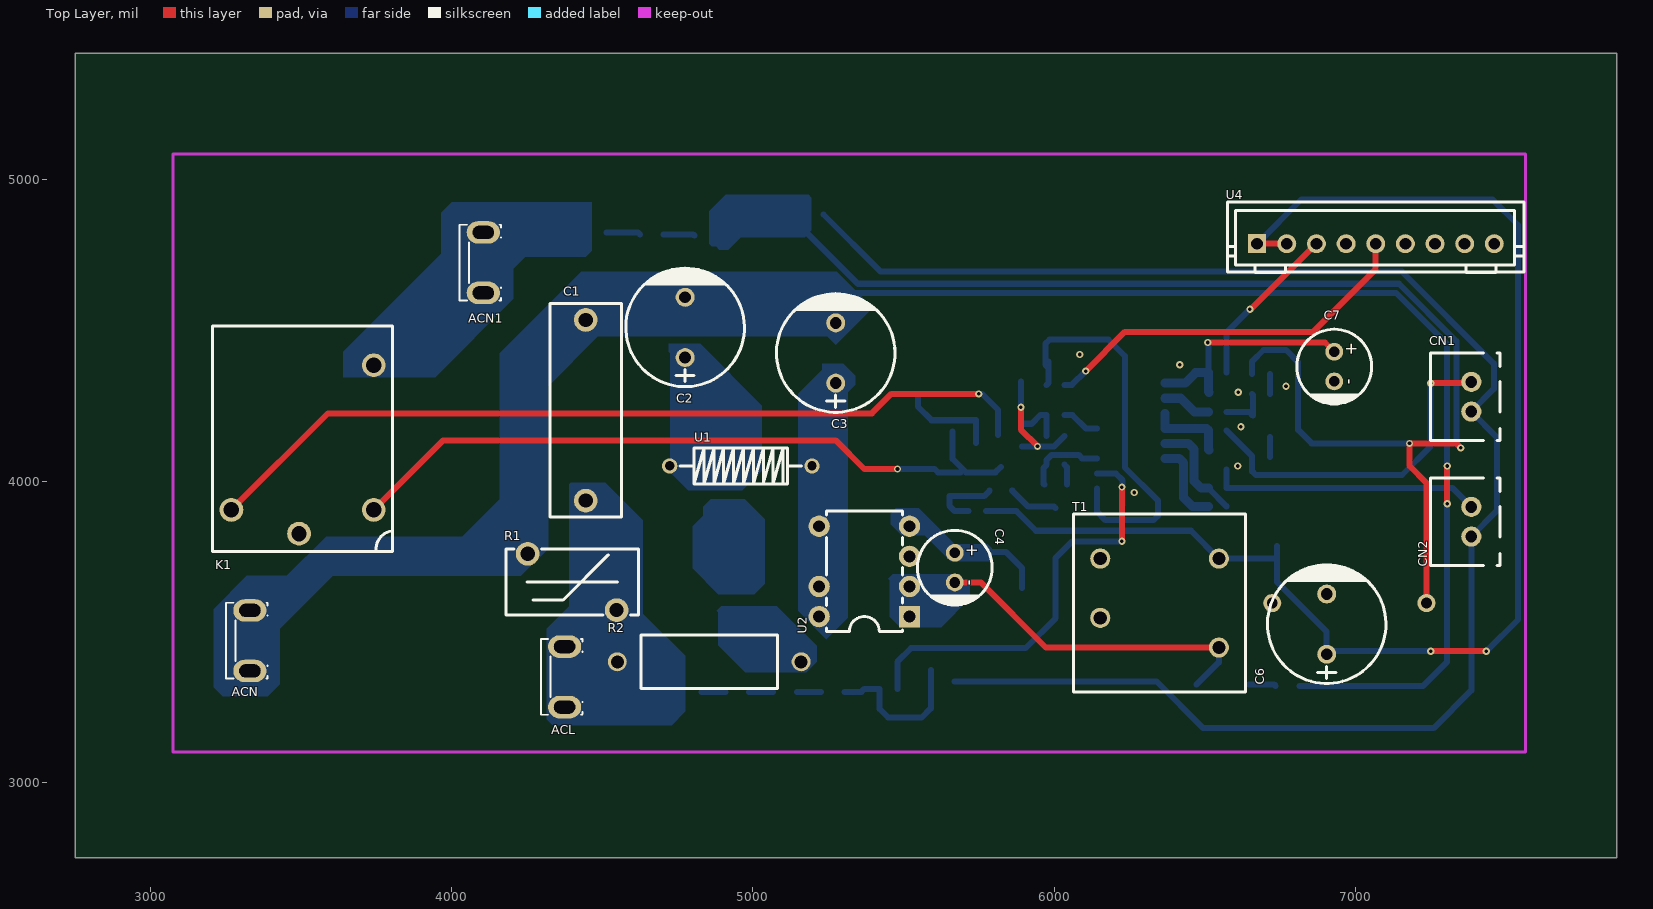
[diagram p0: Top Layer view]
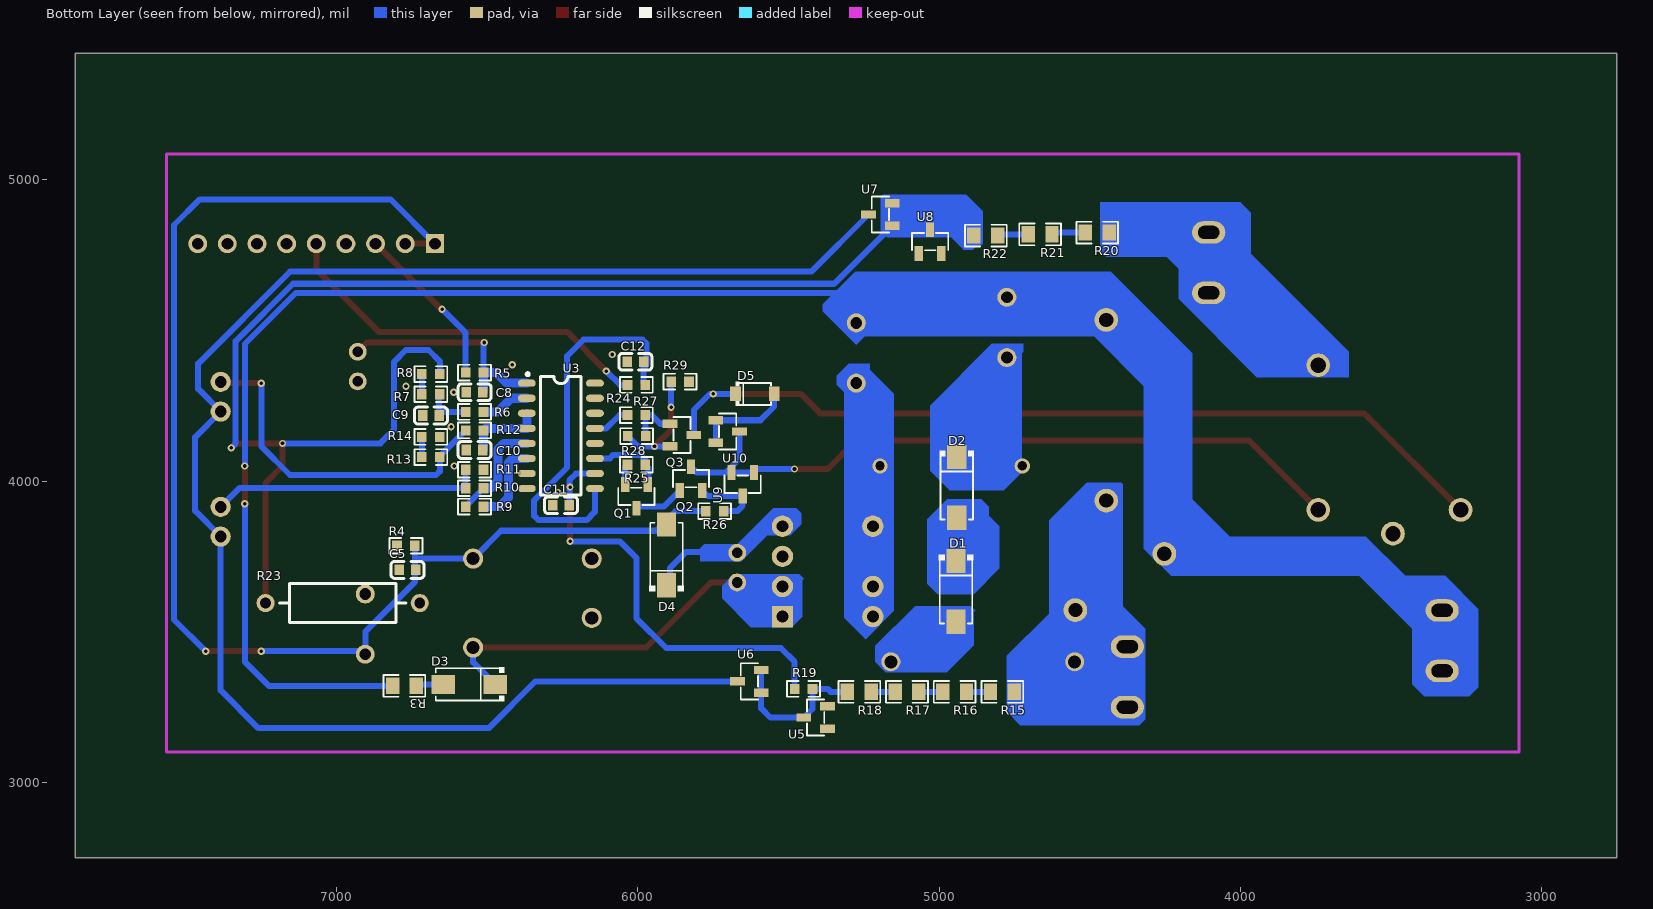
[diagram p1: Bottom Layer view, seen from below]
# Altium PCB MISC51809.pcbdoc
Units mil, origin at the board's own origin, x right, y up, seen from the top; angles counter-clockwise.
Board outline 5118.18 x 2670.55 mil, 2 copper layers (Top Layer, Bottom Layer), stack 62.206 mil thick; 66 components, 45 nets, 171 pads, 23 vias.

## Layer stack, top to bottom
Top Solder Mask Layer: solder mask 0.394, Dk 3.3
Top Layer: signal copper 1.379
Dielectric1: surface 59.449, FR4, Dk 4.5
Bottom Layer: signal copper 1.378
Bottom Solder Mask Layer: solder mask 0.394, Dk 3.3

## Board outline
7868.18,2750 2750,2750 2750,5420.55 7868.18,5420.55

## Design rules (kind name [scope] priority, off if disabled: settings)
BoardOutlineClearance copperThickness2oz_1 [All] p2 off: genericclearance=7.99 ignorepadtopadclearanceinfootprint=FALSE except(0: Arc-SplitContinuation Track-SplitContinuation SMDPad-SplitContinuation THPad-SplitContinuation Via-SplitContinuation Fill-SplitContinuation Region-SplitContinuation Poly-SplitContinuation Text-SplitContinuation Hole-SplitContinuation; 5.98: Arc-CutoutEdge SMDPad-CutoutEdge THPad-CutoutEdge Via-CutoutEdge Fill-CutoutEdge Region-CutoutEdge Text-CutoutEdge; 6.93: Hole-OutlineEdge Hole-CutoutEdge; 10: Poly-OutlineEdge Poly-CutoutEdge; 11.81: Arc-OutlineEdge Track-OutlineEdge SMDPad-OutlineEdge THPad-OutlineEdge Via-OutlineEdge Fill-OutlineEdge Region-OutlineEdge Text-OutlineEdge Track-CutoutEdge)
BoardOutlineClearance copperThickness1oz_1 [All] p4: genericclearance=4.02 ignorepadtopadclearanceinfootprint=FALSE except(0: Arc-SplitContinuation Track-SplitContinuation SMDPad-SplitContinuation THPad-SplitContinuation Via-SplitContinuation Fill-SplitContinuation Region-SplitContinuation Poly-SplitContinuation Text-SplitContinuation Hole-SplitContinuation; 6: SMDPad-CutoutEdge THPad-CutoutEdge Via-CutoutEdge Fill-CutoutEdge Region-CutoutEdge Text-CutoutEdge; 6.93: Hole-OutlineEdge Hole-CutoutEdge; 10: Poly-OutlineEdge Poly-CutoutEdge; 11.8: Arc-OutlineEdge Track-OutlineEdge SMDPad-OutlineEdge THPad-OutlineEdge Via-OutlineEdge Fill-OutlineEdge Region-OutlineEdge Text-OutlineEdge; 11.81: Arc-CutoutEdge Track-CutoutEdge)
Clearance copperThickness2oz [All] p1 off: gap=7.99 ignorepadtopadclearanceinfootprint=FALSE except(5.98: SMDPad-Track SMDPad-SMDPad THPad-Track SMDPad-THPad THPad-THPad Track-Via SMDPad-Via THPad-Via Via-Via Fill-Track Region-Track Fill-SMDPad Region-SMDPad Fill-THPad Region-THPad Fill-Via Region-Via Fill-Fill Fill-Region Region-Region Arc-Track Arc-SMDPad Arc-THPad Arc-Via Fill-Arc Region-Arc Arc-Arc Text-Track SMDPad-Text Text-THPad Text-Via Fill-Text Region-Text Arc-Text Text-Text; 6.93: Hole-Track Hole-SMDPad Hole-THPad Hole-Via Fill-Hole Region-Hole Hole-Arc Hole-Text; 10: Poly-Track Poly-SMDPad Poly-THPad Poly-Via Poly-Fill Poly-Region Poly-Poly Poly-Arc Poly-Text Poly-Hole)
Clearance copperThickness1oz [All] p3: gap=4.02 ignorepadtopadclearanceinfootprint=FALSE except(5.98: SMDPad-Track SMDPad-SMDPad THPad-Track SMDPad-THPad THPad-THPad Track-Via SMDPad-Via THPad-Via Via-Via Fill-Track Region-Track Fill-SMDPad Region-SMDPad Fill-THPad Region-THPad Fill-Via Region-Via Fill-Fill Fill-Region Region-Region; 6: Arc-Track Arc-SMDPad Arc-THPad Arc-Via Fill-Arc Region-Arc Arc-Arc Text-Track SMDPad-Text Text-THPad Text-Via Fill-Text Region-Text Arc-Text Text-Text; 6.93: Hole-Track Hole-SMDPad Hole-THPad Hole-Via Fill-Hole Region-Hole Hole-Arc Hole-Text; 10: Poly-Track Poly-SMDPad Poly-THPad Poly-Via Poly-Fill Poly-Region Poly-Poly Poly-Arc Poly-Text Poly-Hole)
DiffPairsRouting differentialPair [All] p1: maxlimit=6 minlimit=6 mostfreqgap=6 toplayer_minwidth=5 toplayer_prefwidth=10 toplayer_maxwidth=100 toplayer_mingap=6 toplayer_prefgap=6 toplayer_maxgap=6 bottomlayer_minwidth=5 bottomlayer_prefwidth=10 bottomlayer_maxwidth=100 bottomlayer_mingap=6 bottomlayer_prefgap=6 bottomlayer_maxgap=6 maxuncoupledlength=10
HoleToHoleClearance otherClearance [All] p1: gap=11.81 allowstackedmicrovias=TRUE
Length netLength [All] p1: minlimit=0 maxlimit=0
MatchedLengths netLengthTolerance [All] p1: tolerance=1000
PasteMaskExpansion pasteMaskExpansion [All] p1: expansion=0
PlaneConnect innerPlane [All] p1: planeconnectstyle=Relief reliefexpansion=20 reliefentries=4 reliefconductorwidth=10 reliefairgap=10
PolygonConnect copperRegion [(InNet('GND'))] p1: connectstyle=Relief reliefconductorwidth=10 reliefentries=4 polygonreliefangle="90 Angle" airgapwidth=10 via.connectstyle=Relief via.reliefconductorwidth=10 via.reliefentries=4 via.polygonreliefangle="90 Angle" via.airgapwidth=10
RoutingVias viaSize [All] p1: holewidth=12.01 width=24.02 viastyle="Through Hole" minholewidth=11.81 minwidth=19.68 maxholewidth=248.03 maxwidth=393.7
SolderMaskExpansion solderMaskExpansion [IsVia] p1: expansion=-1000 istentingtop=TRUE
SolderMaskExpansion solderMaskExpansion [All] p2: expansion=2 istentingtop=FALSE
Width copperThickness2oz_2 [All] p1 off: maxlimit=100 minlimit=8 preferedwidth=10
Width copperThickness1oz_2 [All] p2: maxlimit=100 minlimit=5 preferedwidth=10

## Components (designator, comment, footprint, x,y, rotation, side; value= is the part's Value field where it differs from the comment)
ACL "T250036-3B80" CONN-TH_XFCN-T250036-3B80 4375,3350 r90 top
ACN "T250036-3B80" CONN-TH_XFCN-T250036-3B80 3330,3470 r90 top
ACN1 "T250036-3B80" CONN-TH_XFCN-T250036-3B80 4105,4725 r90 top
C1 "100nF" CAP-TH_L18.0-W6.0-P15.00-D1.2 4445,4235 r270 top
C2 "4.7uF" CAP-TH_BD10.0-P5.00-D1.0-FD 4775,4510 r90 top
C3 "4.7uF" CAP-TH_BD10.0-P5.00-D1.0-FD 5275,4425 r90 top
C4 "4.7uF" CAP-TH_BD6.3-P2.50-D0.5-FD 5670.39,3712.57 r270 top
C5 "100nF" C0603 6765,3705 r180 bottom
C6 "470uF" CAP-TH_BD10.0-P5.00-D1.0-FD 6905,3525 r90 top
C7 "100uF" CAP-TH_BD6.3-P2.50-D0.5-FD 6930,4380 r270 top
C8 "1uF" C0603 6542.2,4294.74 r0 bottom
C9 "1uF" C0603 6687.19,4217.32 r0 bottom
C10 "100nF" C0603 6542.2,4102.89 r180 bottom
C11 "100nF" C0603 6255.14,3919.92 r180 bottom
C12 "100nF" C0603 6008.36,4396.02 r0 bottom
CN1 "B2B-XH-A(LF)(SN)" CONN-TH_B2B-XH-A-LF-SN 7385,4280 r90 top
CN2 "B2B-XH-A(LF)(SN)" CONN-TH_B2B-XH-A-LF-SN 7385,3865 r90 top
D1 "US1M" SMA_L4.4-W2.8-LS5.4-RD 4943.88,3633.69 r270 bottom
D2 "US1M" SMA_L4.4-W2.8-LS5.4-RD 4941.31,3978.88 r270 bottom
D3 "BYV26C" SMA_L4.4-W2.6-LS5.1-FD 6560,3325 r180 bottom
D4 "US1M" SMA_L4.4-W2.8-LS5.4-RD 5905,3755 r90 bottom
D5 "MMSZ5242B" SOD-123_L2.7-W1.6-LS3.7-RD 5611.93,4289.41 r180 bottom
K1 "HF3FF-012-1HST" RELAY-TH_HF3FF-012-1HST 3505,4105 r90 top
Q1 "SS8050" SOT-23-3_L2.9-W1.3-P1.90-LS2.4-BR 6004.88,3949.17 r90 bottom
Q2 "SS8050" SOT-23-3_L2.9-W1.3-P1.90-LS2.4-BR 5823.65,4007.83 r270 bottom
Q3 "SS8050" SOT-23-3_L2.9-W1.3-P1.90-LS2.4-BR 5853.65,4152.83 r0 bottom
R1 "180pF" RES-TH_L11.0-W5.5-P7.50-D0.8-S4.70 4400,3665 r0 top
R2 "2.2kΩ" RES-TH_BD4.5-L11.5-P15.50-D0.8 4855,3400 r0 top
R3 "0Ω" R0805 6775,3320 r0 bottom
R4 "10kΩ" R0603 6770,3785 r180 bottom
R5 "1kΩ" R0603 6542.2,4360 r0 bottom
R6 "1kΩ" R0603 6542.2,4229.47 r0 bottom
R7 "1kΩ" R0603 6687.19,4288.2 r0 bottom
R8 "10kΩ" R0603 6687.19,4355.13 r180 bottom
R9 "1kΩ" R0603 6542.2,3915 r0 bottom
R10 "10kΩ" R0603 6542.2,3976.32 r180 bottom
R11 "5.1kΩ" R0603 6542.2,4037.63 r180 bottom
R12 "10kΩ" R0603 6542.2,4168.16 r180 bottom
R13 "5.1kΩ" R0603 6687.19,4079.51 r0 bottom
R14 "1kΩ" R0603 6687.19,4146.44 r0 bottom
R15 "240kΩ" R0805 4790,3300 r0 bottom
R16 "240kΩ" R0805 4948.33,3300 r0 bottom
R17 "240kΩ" R0805 5106.67,3300 r0 bottom
R18 "240kΩ" R0805 5265,3300 r0 bottom
R19 "10kΩ" R0603 5450,3310 r0 bottom
R20 "150kΩ" R0805 4475,4825 r0 bottom
R21 "150kΩ" R0805 4664.52,4819.03 r0 bottom
R22 "180kΩ" R0805 4845,4815 r0 bottom
R23 "4.7kΩ" RES-TH_BD3.3-L9.0-P13.00-D0.6 6980,3595 r180 bottom
R24 "100Ω" R0603 6004.88,4319.17 r180 bottom
R25 "4.7K" R0603 6004.88,4054.17 r0 bottom
R26 "4.7K" R0603 5745,3900 r0 bottom
R27 "4.7kΩ" R0603 6004.88,4219.17 r0 bottom
R28 "4.7kΩ" R0603 6004.04,4149.24 r180 bottom
R29 "10kΩ" R0603 5860,4330 r0 bottom
T1 "XREE14-250408" XFMR-TH_XREE14-250408 6350,3595 r0 top
U1 "1mH" IND-TH_BD3.0-L8.0-P12.00-D0.6 4960,4050 r0 top
U2 "PN8034NSC-T1" DIP-8_7P-L9.3-W6.4-P2.54-LS7.6-BL-PE6 5370,3700 r90 top
U3 "CMS79F123" SOPN-16_L9.9-W3.9-P1.27-LS6.0-BL 6255.65,4149.93 r270 bottom
U4 "ZX-XH2.54-9PZZ" CONN-TH_9P-P2.50_ZX-XH2.54-9PZZ 7067.69,4787.85 r0 top
U5 "MMBD4148" SOT-23-3_L2.9-W1.3-P1.90-LS2.4-BR 5410,3215 r180 bottom
U6 "MMBD4148" SOT-23-3_L2.9-W1.3-P1.90-LS2.4-BR 5630,3335 r180 bottom
U7 "MMBD4148" SOT-23-3_L2.9-W1.3-P1.90-LS2.4-BR 5195,4885 r180 bottom
U8 "MMBD4148" SOT-23-3_L2.9-W1.3-P1.90-LS2.4-BR 5030,4795 r270 bottom
U9 "MMBD4148" SOT-23-3_L2.9-W1.3-P1.90-LS2.4-BR 5651.93,3989.41 r90 bottom
U10 "MMBD4148" SOT-23-3_L2.9-W1.3-P1.90-LS2.4-BR 5701.93,4164.41 r0 bottom

## Footprints (in the part's own frame and the unit in brackets; to place one, negate y for a bottom-side part, rotate by r counter-clockwise, add the part's x,y. Pads: shape width x height; smd on the part's side, far side on the other; paste and mask are expansions set on the pad)
C0603 [mm]
  rect 0.8x0.9 smd: 1(-0.7,0) 2(0.7,0)
  silkscreen extent -1.39,-0.71 1.39,0.71
CAP-TH_BD6.3-P2.50-D0.5-FD [mm]
  round 1.5 hole 0.9 paste+0 mask+0.05: 1(-1.25,0) 2(1.25,0)
  silkscreen extent -3.15,-3.15 3.21,3.15
CAP-TH_BD10.0-P5.00-D1.0-FD [mm]
  round 1.6 hole 1: 1(-2.54,0) 2(2.54,0)
  silkscreen extent -5,-5 5.08,5
CAP-TH_L18.0-W6.0-P15.00-D1.2 [mm]
  round 2 hole 1.2: 1(-7.62,0) 2(7.62,0)
  silkscreen extent -9,-3 9,3
CONN-TH_9P-P2.50_ZX-XH2.54-9PZZ [mm]
  rect 1.524x1.6 hole 1: 1(-10,0)
  round 1.6 hole 1: 2(-7.5,0) 3(-5,0) 4(-2.5,0) 5(0,0) 6(2.5,0) 7(5,0) 8(7.5,0) 9(10,0)
  silkscreen extent -12.5,-2.41 12.5,3.5
CONN-TH_B2B-XH-A-LF-SN [mm]
  round 1.7 hole 1: 1(1.25,0) 2(-1.25,0)
  silkscreen extent -3.68,-2.41 3.68,3.43
CONN-TH_XFCN-T250036-3B80 [mm]
  oval 1.9x2.8 hole 1.1 slot 1.8 at 90 deg: 1(-2.55,0) 2(2.55,0)
  silkscreen extent -3.2,-1.5 3.2,2
DIP-8_7P-L9.3-W6.4-P2.54-LS7.6-BL-PE6 [mm]
  rect 1.8x1.8 hole 1: 1(-3.81,-3.81)
  round 1.8 hole 1: 2(-1.27,-3.81) 3(1.27,-3.81) 4(3.81,-3.81) 5(3.81,3.81) 6(-1.27,3.81) 7(-3.81,3.81)
  silkscreen extent -5.08,-3.2 5.08,3.2
IND-TH_BD3.0-L8.0-P12.00-D0.6 [mm]
  round 1.3 hole 0.8 paste+0 mask+0.05: 1(-6,0) 2(6,0)
  silkscreen extent -5.12,-1.5 5.12,1.5
R0603 [mil]
  rect 31.75x34.02 smd paste-3937.01 mask+2: 1(-29.66,0) 2(29.66,0)
  silkscreen extent -55,-26 55,26
R0805 [mm]
  rect 1.133x1.377 smd paste-100 mask+0.051: 1(-1,0) 2(1,0)
  silkscreen extent -1.76,-0.92 1.76,0.92
RELAY-TH_HF3FF-012-1HST [mm]
  round 2 hole 1.3: 1(-5.1,-6) 2(-7.1,0.3) 3(7.1,-6) 4(-5.1,6)
  silkscreen extent -8.6,-7.6 10.4,7.6
RES-TH_BD3.3-L9.0-P13.00-D0.6 [mil]
  round 60 hole 36: 1(-255.91,0) 2(255.9,0)
  silkscreen extent -210,-65 210,65
RES-TH_BD4.5-L11.5-P15.50-D0.8 [mm]
  round 1.6 hole 1.1: 1(-7.75,0) 2(7.75,0)
  silkscreen extent -5.75,-2.26 5.75,2.25
RES-TH_L11.0-W5.5-P7.50-D0.8-S4.70 [mm]
  round 2 hole 1.2: 1(-3.75,2.375) 2(3.75,-2.375)
  silkscreen extent -5.59,-2.79 5.59,2.79
SMA_L4.4-W2.6-LS5.1-FD [mm]
  rect 2x1.62 smd: 1(-2.2,0) 2(2.2,0)
  silkscreen extent -2.81,-1.44 2.97,1.44
SMA_L4.4-W2.8-LS5.4-RD [mil]
  rect 80.57x63.78 smd: 1(-101,0) 2(101,0)
  silkscreen extent -121,-57 106,57
SOD-123_L2.7-W1.6-LS3.7-RD [mm]
  rect 0.91x1.22 smd: 1(-1.635,0) 2(1.635,0)
  silkscreen extent -1.6,-1 1.38,1
SOPN-16_L9.9-W3.9-P1.27-LS6.0-BL [mm]
  oval 0.6x1.508 smd: 1(-4.445,-2.873) 2(-3.175,-2.873) 3(-1.905,-2.873) 4(-0.635,-2.873) 5(0.635,-2.873) 6(1.905,-2.873) 7(3.175,-2.873) 8(4.445,-2.873) 9(4.445,2.873) 10(3.175,2.873) 11(1.905,2.873) 12(0.635,2.873) 13(-0.635,2.873) 14(-1.905,2.873) 15(-3.175,2.873) 16(-4.445,2.873)
  silkscreen extent -5.33,-2.93 5,1.7
SOT-23-3_L2.9-W1.3-P1.90-LS2.4-BR [mm]
  rect 1.25x0.7 smd: 1(1,-0.95) 2(1,0.95) 3(-1,0)
  silkscreen extent -0.73,-1.53 0.73,1.53
XFMR-TH_XREE14-250408 [mm]
  round 1.7 hole 1.1: 1(-5,3.75) 3(-5,-1.25) 5(5,-3.75) 8(5,3.75)
  silkscreen extent -7.24,-7.49 7.24,7.49

## Via types
v1: diameter 24.02, hole 12, Top Layer to Bottom Layer, 23 vias

## Nets (pads, with @x,y where several pads share a name; then routed paths per layer and width w, separated by ;. In a path a pad name is that pad's centre, name@x,y a point inside that pad or via, vN(x,y) a via of type N, cw(c..) or ccw(c..) an arc to the next point about the centre after c; other vN are vias at no path point)
$1N3: D1.2 R2.2
$1N4: D1.1 D2.2
$1N5: C2.1 D2.1 U1.1
$1N6: C3.1 U1.2 U2.5 U2.6 U2.7
$1N7: C4.2 D3.2 T1.5 U2.1 U2.2 | length 1118.7
  Top Layer w20: C4.2 5756.64,3663.36 5972.64,3447.36 T1.5
  Bottom Layer w20: D3.2 6546.85,3398.46 T1.5
$1N8: C4.1 D4.1 U2.4 | length 227.4
  Bottom Layer w20: 5755,3765 5840,3765 5894,3711 D4.1@5894,3645
$1N9: D3.1 R3.1 | length 91.1
  Bottom Layer w20: D3.1 6730.63,3325 R3.1
$1N14: R5.2 U4.3 | length 553.4
  Top Layer w20: v1(6650,4570) 6652.98,4570 U4.3
  Bottom Layer w20: R5.2 6571.86,4491.86 v1(6650,4570)
$1N15: C7.1 C8.1 R5.1 U3.1 | length 758.2
  Top Layer w20: v1(6510,4460) 6899.21,4460 C7.1
  Bottom Layer w20: v1(6510,4460) 6512.54,4457.46 R5.1
  Bottom Layer w30: U3.1 6434.93,4324.93 6470,4360 R5.1 6512.54,4296.84 C8.1
$1N16: R6.1 U3.2 | length 162.6
  Bottom Layer w30: U3.2 6420.07,4274.93 6465.53,4229.47 R6.1
$1N17: C9.1 R6.2 R7.1 | length 164.6
  Bottom Layer w20: R6.2 6647.48,4229.47 C9.1 6659.63,4286.1 R7.1
$1N20: R7.2 R8.1 | length 66.9
  Bottom Layer w20: R7.2 R8.1
$1N22: C10.2 R12.2 U3.3 U3.4 | length 262.7
  Bottom Layer w30: U3.3 U3.4 6505.76,4174.93 R12.2 6512.54,4105 C10.2
$1N25: R9.2 R10.2 U3.5 | length 352.7
  Bottom Layer w20: R10.2 6571.86,3917 R9.2
  Bottom Layer w30: U3.5 6445.07,4124.93 6465,4105 6465,4000 6488.68,3976.32 R10.2
$1N26: R9.1 U3.6 | length 277.4
  Bottom Layer w30: U3.6 6415.07,4074.93 6430,4060 6430,3945 6460,3915 R9.1
$1N27: CN2.1 R10.1 R11.1 | length 900.2
  Bottom Layer w20: R11.1 R10.1 7322.9,3976.32 CN2.1
$1N31: CN1.1 R12.1 R13.1 | length 1154.9
  Top Layer w20: v1(7250,4325) 7380.79,4325 CN1.1
  Bottom Layer w20: R12.1 6657.53,4082.48 R13.1 6657.53,4032.47 6670,4020 7155,4020 7250,4115 v1(7250,4325)
$1N32: R13.2 R14.2 | length 66.9
  Bottom Layer w20: R13.2 R14.2
$1N35: R15.2 R16.1 | length 79.6
  Bottom Layer w20: R15.2 R16.1
$1N36: R16.2 R17.1 | length 79.6
  Bottom Layer w20: R16.2 R17.1
$1N37: R17.2 R18.1 | length 79.6
  Bottom Layer w20: R17.2 R18.1
$1N39: R18.2 R19.1 U5.3 U6.1 U6.2 | length 507.9
  Bottom Layer w20: R18.2 5360,3300 5370,3310 R19.1 5420.34,3244.03 U5.3 5560,3215 5590.63,3245.63 U6.1 U6.2
$1N54: R20.2 R21.1 | length 113.3
  Bottom Layer w20: R20.2 4619.17,4825 R21.1
$1N55: R21.2 R22.1 | length 103.4
  Bottom Layer w20: R21.2 4801.6,4819.03 R22.1
$1N56: ACN1.1 ACN1.2 K1.3 R20.1
$1N57: C12.1 R24.2 U3.9 | length 1327.7
  Bottom Layer w20: R24.2 5980.8,4324.76 5980.8,4376.59 ; C12.1 5980.8,4376.59 ; U3.9 6142.54,3897.46 6170,3870 6330,3870 6344.14,3884.14 6344.14,3935.86 6235,4045 6235,4415 6180,4470 5985,4470 5970.86,4455.86 5970.86,4386.53 5980.8,4376.59
$1N60: Q1.2 R25.2 | length 68.8
  Bottom Layer w20: R25.2 6042.28,4046.43 Q1.2
$1N61: Q1.1 R25.1 U3.11 | length 266.3
  Bottom Layer w20: Q1.1 5965,3991.02 5965,4043.96 R25.1 5975.22,4070.22 5992.17,4087.17 6081.19,4087.17 6093.42,4074.93 U3.11
$1N63: Q1.3 Q2.1 | length 168.1
  Bottom Layer w20: Q2.1 5914.51,3915 5999.68,3915 Q1.3
$1N64: Q2.2 R26.1 U9.3 | length 244.8
  Bottom Layer w20: R26.1 5670,3900 5651.93,3918.07 U9.3 5767.84,3950.04 Q2.2
$1N66: K1.1 Q2.3 U9.1 U9.2 U10.3 | length 2365.7
  Top Layer w20: K1.1 3972.01,4135 5275,4135 5370,4040 v1(5480,4040)
  Bottom Layer w20: v1(5480,4040) 5603.31,4040 U9.1 U9.2 ; U10.3 5662.56,4073.71 5707.49,4028.78 5805.24,4028.78 Q2.3
$1N67: D5.2 U10.1 U10.2 | length 329.4
  Bottom Layer w20: D5.2 5547.56,4247.44 5593.19,4201.81 U10.1 U10.2
$1N68: D5.1 K1.4 Q3.3 | length 2883.9
  Top Layer w20: K1.4 3589.57,4225 5395,4225 5459.41,4289.41 v1(5750,4289.41)
  Bottom Layer w20: D5.1 5760.59,4289.41 5814.28,4235.72 Q3.3
$1N70: R27.2 U3.13 | length 126.3
  Bottom Layer w20: R27.2 6060.83,4219.17 6105.07,4174.93 U3.13
$1N72: Q3.1 R27.1 R28.2 | length 164.5
  Bottom Layer w20: Q3.1 5925.23,4190.23 5954.17,4219.17 R27.1 5975.22,4150.08 R28.2
$1N73: Q3.2 R28.1 R29.2 | length 392.6
  Top Layer w20: v1(5889.66,4245) 5889.66,4170.34 v1(5945,4115)
  Bottom Layer w20: v1(5889.66,4245) R29.2 ; Q3.2 5999.89,4115.43 R28.1
$1N78: U4.7
+12V: C5.2 C6.1 D4.2 R4.2 R26.2 T1.8 U4.1 U4.2 | length 4512.3
  Top Layer w20: U4.1 U4.2 ; v1(7250,3435) v1(7435,3435)
  Bottom Layer w20: R26.2 5875,3900 5940,3835 6454.49,3835 T1.8 6740.34,3742.64 ; U4.1 6821.13,4935 7455,4935 7540,4850 7540,3540 v1(7435,3435) ; R4.2 6740.34,3742.64 ; v1(7250,3435) 6915,3435 C6.1 6905,3500 6740.34,3664.66 6740.34,3742.64
ACL: ACL.1 ACL.2 C1.2 R1.2 R2.1 R15.1
ACN: ACN.1 ACN.2 C1.1 C2.2 C3.2 R1.1 R3.2 | length 3649.2
  Top Layer w20: v1(7305,3925) v1(7305,4050)
  Bottom Layer w20: 5305,4625 7135,4625 7305,4455 v1(7305,4050) ; R3.2 7225,3320 7305,3400 v1(7305,3925)
CN102_5: R24.1 U4.5 | length 1277.2
  Top Layer w20: v1(6105,4365) 6235,4495 6860,4495 7067.69,4702.69 U4.5
  Bottom Layer w20: R24.1 6059.17,4319.17 v1(6105,4365)
GND: C5.1 C6.2 C7.2 C8.2 C9.2 C10.1 C11.1 C12.2 R4.1 R11.2 R14.1 R23.2 R29.1 U3.16 U4.4 U4.8 U5.1 U5.2 U8.1 U8.2
  other v1: 6266.17,3962.13 6610,4050 6620,4180 6611.33,4294.74 6770,4315 6417.37,4386.01 6085,4420
J_D143: R8.2 R22.2 R23.1 U7.1 U7.2 U8.3 | length 4269
  Top Layer w20: R23.1 7235.9,3994.09 7180,4050 v1(7180,4125) 7335,4125 v1(7350,4110)
  Bottom Layer w20: U7.1 5348.23,4655 7145,4655 7335.55,4464.45 7335.55,4124.45 v1(7350,4110) ; R8.2 6657.53,4397.53 6695,4435 6770,4435 6810,4395 6810,4170 6855,4125 v1(7180,4125)
MCU_VDD: CN1.2 CN2.2 U6.3 U7.3 | length 5448.8
  Bottom Layer w20: U7.3 5424.37,4695 7155,4695 7460,4390 7460,4305.79 CN1.2 7470,4145.79 7470,3900.79 CN2.2 7385,3305 7260,3180 6495,3180 6340,3335 U6.3
PA5: C11.2 R19.2 U3.10 | length 1474.8
  Top Layer w20: v1(6225,3800) v1(6225,3980)
  Bottom Layer w20: R19.2 5479.66,3399.66 5525,3445 5905,3445 6005,3545 6005,3745 6060,3800 v1(6225,3800) ; U3.10 6205.07,4024.93 6227.58,4002.42 C11.2
pads on no net: K1.2 T1.1 T1.3 U2.3 U3.7 U3.8 U3.12 U3.14 U3.15 U4.6 U4.9

## Keep-outs
Board Outline Layer:
  lines w10: 3075,3100 3075,5085 7565,5085 7565,3100 3075,3100

## Other copper
Bottom Layer:
  region net ACL: 4390,3990 4395,3995 4510,3995 4635,3870 4635,3560 4775,3420 4775,3235 4730,3190 4335,3190 4315,3210 4315,3510 4390,3585
  region net ACN: 3430,3510 3430,3325 3390,3285 3240,3285 3210,3315 3210,3575 3320,3685 3453.14,3685 3583.14,3815 4035,3815 4160,3940 4160,4425 4430,4695 5277.94,4695 5386.75,4586.19 5386.75,4563.68 5275,4451.92 5246.92,4480 4485,4480 4320,4315 4320,3775 4230,3685 3605,3685
  region net $1N5: 4725,4425 4720,4430 4720,4455 4825,4455 5030,4250 5030,4035 4965,3970 4785,3970 4725,4030
  region net $1N4: 4860,3940 4972.17,3940 5039.64,3872.53 5039.64,3659.64 5005,3625 4885,3625 4800,3710 4800,3850 4835,3885 4835,3915
  region net $1N3: 4895,3585 5080,3585 5212.59,3452.41 5212.59,3399.79 5177.8,3365 4975,3365 4885,3455 4885,3565 4880,3570
  region net $1N6: 5230,4370 5230,4390 5300,4390 5340,4350 5340,4320 5315,4295 5315,3546.41 5244.02,3475.43 5150,3569.44 5150,4290
  region net $1N56: 3640,4430 3965,4755 3965,4890 4000,4925 4465,4925 4465,4765 4445,4745 4245,4745 4205,4705 4205,4605 3945,4345 3640,4345
  region net J_D143: 4855.64,4787.01 4855.64,4895.64 4910,4950 5185,4950 5194.31,4940.69 5194.31,4832.64 5171.67,4810 4960,4810 4918.26,4768.26 4889.04,4768.26 4878.41,4778.89 4863.75,4778.89
  region net $1N7: 5682.96,3690 5720.39,3652.57 5720.39,3610.39 5625,3515 5490,3515 5455,3550 5455,3670 5450,3675 5465,3690
  region net $1N8: 5458.2,3893.74 5474.46,3910 5550,3910 5670,3790 5780,3790 5792.58,3777.42 5792.58,3733.84 5656.16,3733.84 5570,3820 5495,3820 5458.2,3856.8